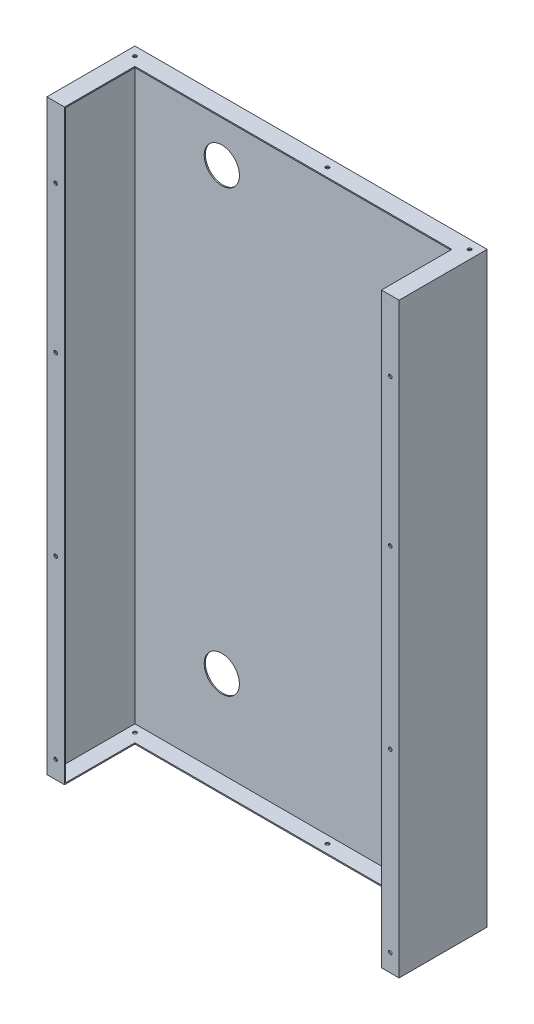
from build123d import *

# Parameters (mm, degrees)
SKETCH_1_W          = 600
SKETCH_1_H          = 150
EXTRUDE_1_DEPTH     = 1000
SHELL_1_T           = -2
SKETCH_3_W          = 596
SKETCH_3_H          = 148
CUT_EXTRUDE_1_DEPTH = 400
SKETCH_4_W          = 28
SKETCH_4_H          = 998
EXTRUDE_2_DEPTH     = 2
SKETCH_5_R          = 30
CUT_EXTRUDE_2_DEPTH = 2
SKETCH_6_W          = 540
SKETCH_6_H          = 120
CUT_EXTRUDE_3_DEPTH = 290
EXTRUDE_3_DEPTH     = 2
SKETCH_8_R          = 3
CUT_EXTRUDE_4_DEPTH = 1118
SKETCH_9_R          = 3
CUT_EXTRUDE_5_DEPTH = 10


with BuildPart() as part:
    # 草图1 → 凸台-拉伸1 (new body)
    with BuildSketch(Plane(origin=(0, 0, 0), x_dir=(1, 0, 0), z_dir=(0, 1, 0))):
        with Locations((300, 75)):
            Rectangle(SKETCH_1_W, SKETCH_1_H)
    extrude(amount=EXTRUDE_1_DEPTH)

    # 抽壳1
    shell_1_openings = [part.faces().sort_by_distance(p)[0] for p in [
        (300, 500, 0),
    ]]
    offset(amount=SHELL_1_T, openings=shell_1_openings, kind=Kind.INTERSECTION)

    # 草图3 → 切除-拉伸1 (cut)
    with BuildSketch(Plane.XZ):
        with Locations((300, -74)):
            Rectangle(SKETCH_3_W, SKETCH_3_H)
    extrude(amount=-CUT_EXTRUDE_1_DEPTH, mode=Mode.SUBTRACT)

    # 草图4 → 凸台-拉伸2 (add)
    with BuildSketch(Plane.XY):
        with Locations((16, 499)):
            Rectangle(SKETCH_4_W, SKETCH_4_H)
        with Locations((584, 499)):
            Rectangle(SKETCH_4_W, SKETCH_4_H)
    extrude(amount=-EXTRUDE_2_DEPTH)

    # 草图5 → 切除-拉伸2 (cut)
    with BuildSketch(Plane(origin=(0, 0, -150), x_dir=(-1, 0, 0), z_dir=(0, 0, -1))):
        with Locations((-150, 150)):
            Circle(SKETCH_5_R)
        with Locations((-150, 900)):
            Circle(SKETCH_5_R)
    extrude(amount=-CUT_EXTRUDE_2_DEPTH, mode=Mode.SUBTRACT)

    # 草图6 → 切除-拉伸3 (cut)
    with BuildSketch(Plane(origin=(0, 1000, 0), x_dir=(1, 0, 0), z_dir=(0, 1, 0))):
        with Locations((300, 60)):
            Rectangle(SKETCH_6_W, SKETCH_6_H)
    extrude(amount=-CUT_EXTRUDE_3_DEPTH, mode=Mode.SUBTRACT)

    # 草图7 → 凸台-拉伸3 (add)
    with BuildSketch(Plane.XZ):
        Polygon((0, 0), (0, -150), (600, -150), (600, 0), (570, 0), (570, -120), (30, -120), (30, 0), align=None)
    extrude(amount=-EXTRUDE_3_DEPTH)

    # 草图8 → 切除-拉伸4 (cut)
    with BuildSketch(Plane(origin=(0, 1000, 0), x_dir=(1, 0, 0), z_dir=(0, 1, 0))):
        with Locations(Location((15, 135, 0), (0, 0, 90))):
            Circle(SKETCH_8_R)
        with Locations(Location((343, 135, 0), (0, 0, 90))):
            Circle(SKETCH_8_R)
        with Locations(Location((585, 135, 0), (0, 0, 90))):
            Circle(SKETCH_8_R)
    extrude(amount=-CUT_EXTRUDE_4_DEPTH, mode=Mode.SUBTRACT)

    # 草图9 → 切除-拉伸5 (cut)
    with BuildSketch(Plane.XY):
        with Locations((15, 880)):
            Circle(SKETCH_9_R)
        with Locations((15, 30)):
            Circle(SKETCH_9_R)
        with Locations(Location((585, 880, 0), (0, 0, 180))):
            Circle(SKETCH_9_R)
        with Locations((15, 330)):
            Circle(SKETCH_9_R)
        with Locations(Location((585, 630, 0), (0, 0, 180))):
            Circle(SKETCH_9_R)
        with Locations((15, 630)):
            Circle(SKETCH_9_R)
        with Locations(Location((585, 330, 0), (0, 0, 180))):
            Circle(SKETCH_9_R)
        with Locations(Location((585, 30, 0), (0, 0, 180))):
            Circle(SKETCH_9_R)
    extrude(amount=-CUT_EXTRUDE_5_DEPTH, mode=Mode.SUBTRACT)


solid = part.part
